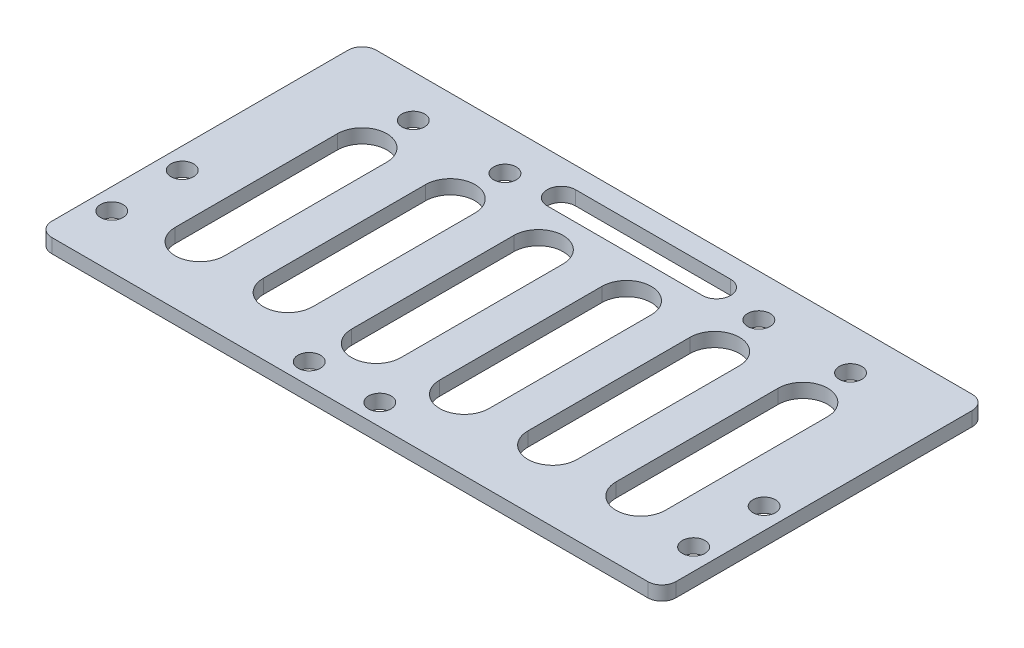
SolidWorks part; units mm, degrees
material "Thornel Mat VMA"
ref_plane "Front Plane" through (0, 0, 0) normal (0, 0, 1) x (1, 0, 0)
ref_plane "Top Plane" through (0, 0, 0) normal (0, 1, 0) x (1, 0, 0)
ref_plane "Right Plane" through (0, 0, 0) normal (1, 0, 0) x (0, 0, -1)
sketch "Sketch1" plane through (0, 0, 0) normal (0, 1, 0) x (1, 0, 0)
  line L0 (0, 23) -> (0, -23) construction
  line L1 (-44.25, 23) -> (44.25, 23)
  line L2 (-44.25, 23) -> (-44.25, -23)
  line L3 (-44.25, -23) -> (44.25, -23)
  line L4 (44.25, 23) -> (44.25, -23)
  line L5 (-44.25, 23) -> (44.25, -23) construction
  line L6 (-44.25, -23) -> (44.25, 23) construction
  line L7 (-41.25, -5.5) -> (-41.25, -15.5) construction
  line L8 (41.25, -5.5) -> (41.25, -15.5) construction
  line L9 (-8.75, -20) -> (1.25, -20) construction
  line L10 (-31, 17) -> (-18, 17) construction
  line L11 (18, 17) -> (31, 17) construction
  line L12 (-44.25, 0) -> (44.25, 0) construction
  line L13 (-8.75, 20) -> (1.25, 20) construction
  circle A0 centre (-41.25, -5.5) radius 1.6
  circle A1 centre (-41.25, -15.5) radius 1.6
  circle A4 centre (41.25, -15.5) radius 1.6
  circle A5 centre (41.25, -5.5) radius 1.6
  circle A6 centre (-8.75, -20) radius 1.6
  circle A7 centre (1.25, -20) radius 1.6
  circle A8 centre (-31, 17) radius 1.6
  circle A9 centre (-18, 17) radius 1.6
  circle A10 centre (18, 17) radius 1.6
  circle A11 centre (31, 17) radius 1.6
  point P0 (0, 0)
  dimension "D1" = 3.2
  dimension "D7" = 3
  dimension "D9" = 13
  dimension "D11" = 3.2
  dimension "D2" = 3
  dimension "D3" = 7.5
  dimension "D4" = 10
  dimension "D5" = 46
  dimension "D6" = 88.5
  dimension "D8" = 35.5
  dimension "D10" = 6
  dimension "D12" = 36
extrude "Boss-Extrude1" add sketch "Sketch1" along normal blind 2
sketch "Sketch2" plane through (0, 2, 0) normal (0, 1, 0) x (1, 0, 0)
  line L0 (0, 23) -> (0, -23) construction
  line L1 (44.25, 23) -> (-44.25, 23) construction
  line L2 (-44.25, -23) -> (44.25, -23) construction
  line L3 (-44.25, -1.5) -> (44.25, -1.5) construction
  line L6 (-31.25, 10) -> (-31.25, -13) construction
  line L7 (-27.75, 10) -> (-27.75, -13)
  line L8 (-34.75, 10) -> (-34.75, -13)
  line L9 (-18.75, 10) -> (-18.75, -13) construction
  line L10 (-15.25, 10) -> (-15.25, -13)
  line L11 (-22.25, 10) -> (-22.25, -13)
  line L12 (-6.25, 10) -> (-6.25, -13) construction
  line L13 (-2.75, 10) -> (-2.75, -13)
  line L14 (-9.75, 10) -> (-9.75, -13)
  line L15 (6.25, 10) -> (6.25, -13) construction
  line L16 (9.75, 10) -> (9.75, -13)
  line L17 (2.75, 10) -> (2.75, -13)
  line L18 (18.75, 10) -> (18.75, -13) construction
  line L19 (22.25, 10) -> (22.25, -13)
  line L20 (15.25, 10) -> (15.25, -13)
  line L21 (31.25, 10) -> (31.25, -13) construction
  line L22 (34.75, 10) -> (34.75, -13)
  line L23 (27.75, 10) -> (27.75, -13)
  line L24 (-44.25, 23) -> (-44.25, -23) construction
  line L27 (44.25, -23) -> (44.25, 23) construction
  line L28 (-11, 18) -> (11, 18) construction
  line L29 (-11, 20) -> (11, 20)
  line L30 (-11, 16) -> (11, 16)
  arc A0 (-27.75, 10) -> (-34.75, 10) centre (-31.25, 10) ccw
  arc A1 (-34.75, -13) -> (-27.75, -13) centre (-31.25, -13) ccw
  arc A2 (-15.25, 10) -> (-22.25, 10) centre (-18.75, 10) ccw
  arc A3 (-22.25, -13) -> (-15.25, -13) centre (-18.75, -13) ccw
  arc A4 (-2.75, 10) -> (-9.75, 10) centre (-6.25, 10) ccw
  arc A5 (-9.75, -13) -> (-2.75, -13) centre (-6.25, -13) ccw
  arc A6 (9.75, 10) -> (2.75, 10) centre (6.25, 10) ccw
  arc A7 (2.75, -13) -> (9.75, -13) centre (6.25, -13) ccw
  arc A8 (22.25, 10) -> (15.25, 10) centre (18.75, 10) ccw
  arc A9 (15.25, -13) -> (22.25, -13) centre (18.75, -13) ccw
  arc A10 (34.75, 10) -> (27.75, 10) centre (31.25, 10) ccw
  arc A11 (27.75, -13) -> (34.75, -13) centre (31.25, -13) ccw
  circle A14 centre (-8.75, -20) radius 1.6 construction
  arc A15 (-11, 20) -> (-11, 16) centre (-11, 18) ccw
  arc A16 (11, 16) -> (11, 20) centre (11, 18) ccw
  point P9 (0, 18)
  point P14 (-31.25, -1.5)
  point P22 (-18.75, -1.5)
  point P29 (-6.25, -1.5)
  point P36 (6.25, -1.5)
  point P43 (18.75, -1.5)
  point P50 (31.25, -1.5)
  dimension "D1" = 3.5
  dimension "D7" = 2
  dimension "D2" = 23
  dimension "D4" = 12.5
  dimension "D5" = 7
  dimension "D6" = 3
  dimension "D8" = 22
  dimension "D3" = 6
extrude "Cut-Extrude1" cut sketch "Sketch2" against normal through all
fillet "Fillet1" radius 2 4 edges at (44.25, 1, -23) (44.25, 1, 23) (-44.25, 1, 23) (-44.25, 1, -23)
